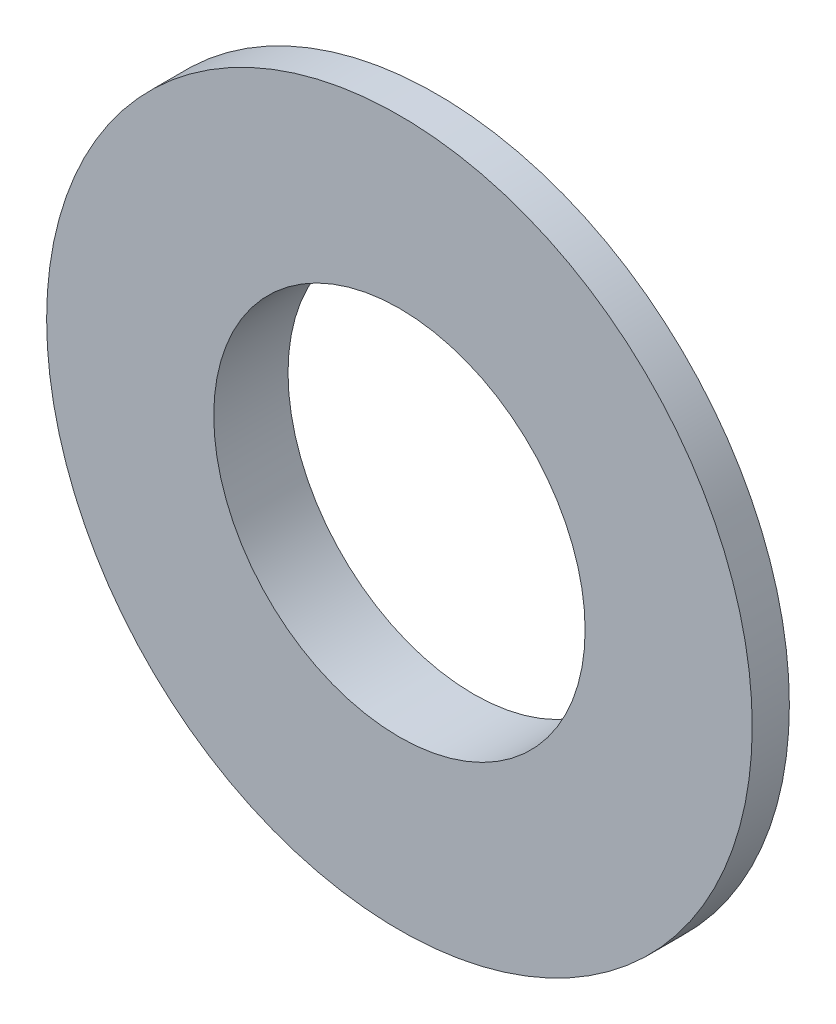
SolidWorks part; units mm, degrees
ref_plane "Front Plane" through (0, 0, 0) normal (0, 0, 1) x (1, 0, 0)
ref_plane "Top Plane" through (0, 0, 0) normal (0, 1, 0) x (1, 0, 0)
ref_plane "Right Plane" through (0, 0, 0) normal (1, 0, 0) x (0, 0, -1)
ref_plane "Plane1" through (0, 234.744, 0) normal (0, 1, 0) x (1, 0, 0)
sketch "Sketch1" plane through (0, 234.744, 0) normal (0, 1, 0) x (1, 0, 0)
  line L0 (546.2306, 388.9984) -> (568.7306, 388.9984)
  line L1 (568.7306, 388.9984) -> (568.7306, 393.9984)
  line L2 (568.7306, 393.9984) -> (554.2306, 398.9984)
  line L3 (554.2306, 398.9984) -> (546.2306, 398.9984)
  line L4 (546.2306, 398.9984) -> (546.2306, 388.9984)
  line L5 (521.2306, 398.9984) -> (521.2306, 388.9984) construction
  dimension "D1" = 25
  dimension "D2" = 33
  dimension "D3" = 47.5
  dimension "D4" = 5
  dimension "D5" = 10
revolve "Revolve1" add sketch "Sketch1" angle 360 about L5
